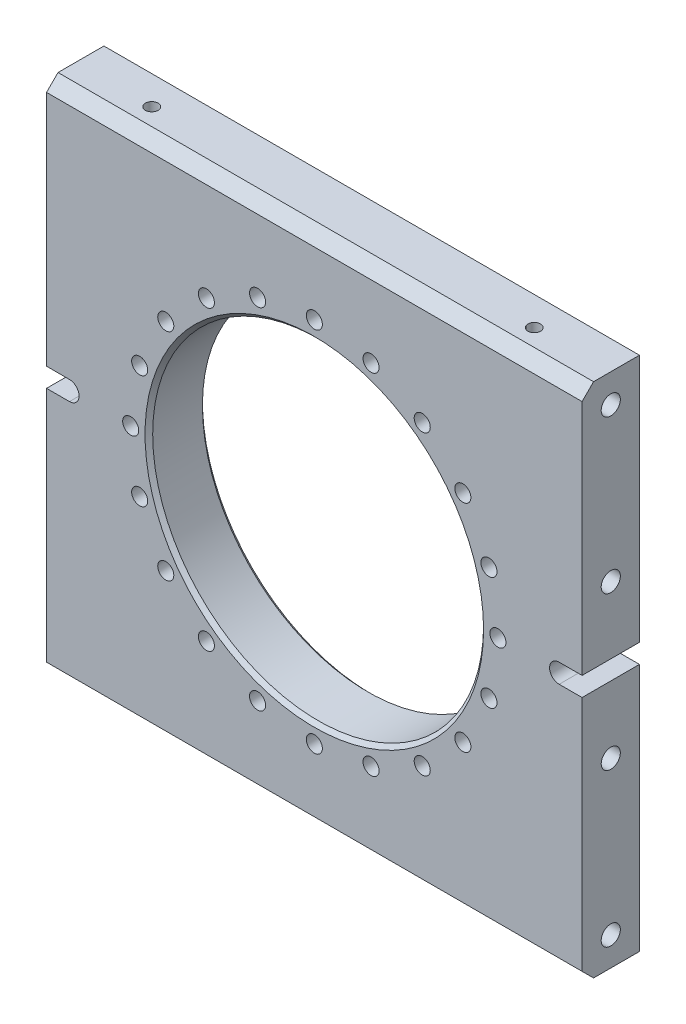
SolidWorks part; units mm, degrees
material "AL6061"
ref_plane "前视基准面" through (0, 0, 0) normal (0, 0, 1) x (1, 0, 0)
ref_plane "上视基准面" through (0, 0, 0) normal (0, 1, 0) x (1, 0, 0)
ref_plane "右视基准面" through (0, 0, 0) normal (1, 0, 0) x (0, 0, -1)
sketch "草图1" plane through (0, 0, 0) normal (0, 0, 1) x (1, 0, 0)
  line L0 (-78.7943, 0) -> (83.5001, 0) construction
  line L1 (0, 54.9642) -> (0, -73.3522) construction
  line L3 (-70, 67.5) -> (70, 67.5)
  line L4 (-70, 67.5) -> (-70, -67.5)
  line L5 (-70, -67.5) -> (70, -67.5)
  line L6 (70, 67.5) -> (70, -67.5)
  circle A0 centre (0, 0) radius 43.25
  dimension "D3" = 86.5
  dimension "D1" = 140
  dimension "D2" = 135
extrude "凸台-拉伸1" add sketch "草图1" along normal mid plane 15
hole_wizard "M6 螺纹孔1" positions "草图2" profile "草图3" tap size "M6" standard "GB"
sketch "草图2" plane through (70, 0, 0) normal (1, 0, 0) x (0, 0, -1)
  line L0 (-10.7947, 0) -> (15.8636, 0) construction
  line L1 (0, 71.0576) -> (0, -73.4981) construction
  point P0 (0, -20)
  point P2 (0, -60)
  point P11 (0, 60)
  point P12 (0, 20)
  dimension "D1" = 40
  dimension "D2" = 120
sketch "草图3" plane through (70, -20, 0) normal (0, 1, 0) x (0, 0, -1)
  line L0 (0, 0) -> (0, 19.5022)
  line L1 (0, 19.5022) -> (2.5, 18)
  line L2 (2.5, 18) -> (2.5, 0)
  line L5 (2.5, 0) -> (0, 0)
  line L10 (0, 19.5022) -> (-2.5, 18) construction
  line L11 (0, -6.35) -> (0, 107.95) construction
  dimension "螺纹孔钻头直径" = 5
  dimension "螺纹孔钻头深度" = 18
  dimension "导头角度" = 118
cosmetic thread "孔螺蚊线1" parameters "D1"=15, "D2"=6
cosmetic thread "孔螺蚊线2" parameters "D1"=15, "D2"=6
cosmetic thread "孔螺蚊线3" parameters "D1"=15, "D2"=6
cosmetic thread "孔螺蚊线4" parameters "D1"=15, "D2"=6
mirror "镜向2" about plane through (0, 0, 0) normal (1, 0, 0) of "M6 螺纹孔1"
hole_wizard "M5 螺纹孔1" positions "草图4" profile "草图5" tap size "M5" standard "GB" end condition through all
sketch "草图4" plane through (0, 0, 7.5) normal (0, 0, 1) x (1, 0, 0)
  line L0 (0, -4.0363) -> (0, 72.7472) construction
  line L1 (0, 0) -> (-73.1227, 0) construction
  circle A0 centre (0, 0) radius 48 construction
  point P0 (0, 48)
  dimension "D1" = 96
sketch "草图5" plane through (0, 48, 7.5) normal (1, 0, 0) x (0, -1, 0)
  line L0 (0, 0) -> (0, 15)
  line L1 (0, 15) -> (2.1, 15)
  line L2 (2.1, 15) -> (2.1, 0)
  line L5 (2.1, 0) -> (0, 0)
  line L11 (0, -6.35) -> (0, 107.95) construction
  dimension "通孔螺纹孔钻头直径" = 4.2
  dimension "通孔螺纹孔钻头深度" = 15
cosmetic thread "孔螺蚊线5" parameters "D2"=5
chamfer "倒角1" distance 1 angle 45 2 edges at (43.25, 0, -7.5) (43.25, 0, 7.5)
pattern_circular "阵列(圆周)1" count 20 over 360 about axis through (0, 0, 0) along (0, 0, 1) of "M5 螺纹孔1"
sketch "草图6" plane through (0, 0, 7.5) normal (0, 0, 1) x (1, 0, 0)
  line L0 (-71.7661, 0) -> (73.0925, 0) construction
  line L1 (0, 70.2589) -> (0, -69.4339) construction
  line L2 (70, -67.5) -> (70, 67.5) construction
  line L3 (70, 2.5) -> (64, 2.5)
  line L4 (70, 2.5) -> (70, -2.5)
  line L5 (70, -2.5) -> (64, -2.5)
  line L7 (-70, -2.5) -> (-64, -2.5)
  line L8 (-70, 2.5) -> (-70, -2.5)
  line L9 (-70, 2.5) -> (-64, 2.5)
  arc A0 (64, 2.5) -> (64, -2.5) centre (64, 0) ccw
  arc A1 (-64, 2.5) -> (-64, -2.5) centre (-64, 0) cw
  dimension "D2" = 6
  dimension "D1" = 5
extrude "切除-拉伸1" cut sketch "草图6" against normal through all
hole_wizard "M4 螺纹孔1" positions "草图7" profile "草图8" tap size "M4" standard "GB"
sketch "草图7" plane through (0, -67.5, 0) normal (0, -1, 0) x (-1, 0, 0)
  line L0 (0, 8.8808) -> (0, -13.9156) construction
  line L1 (-74.1931, 0) -> (74.4728, 0) construction
  point P0 (50, 0)
  point P9 (-50, 0)
  dimension "D1" = 100
sketch "草图8" plane through (-50, -67.5, 0) normal (1, 0, 0) x (0, 0, -1)
  line L0 (0, 0) -> (0, 18.0914)
  line L1 (0, 18.0914) -> (1.65, 17.1)
  line L2 (1.65, 17.1) -> (1.65, 0)
  line L5 (1.65, 0) -> (0, 0)
  line L10 (0, 18.0914) -> (-1.65, 17.1) construction
  line L11 (0, -6.35) -> (0, 107.95) construction
  dimension "螺纹孔钻头直径" = 3.3
  dimension "螺纹孔钻头深度" = 17.1
  dimension "导头角度" = 118
cosmetic thread "孔螺蚊线6" parameters "D1"=15, "D2"=4
cosmetic thread "孔螺蚊线7" parameters "D1"=15, "D2"=4
mirror "镜向3" about plane through (0, 0, 0) normal (0, 1, 0) of "M4 螺纹孔1"
chamfer "倒角2" distance 3 angle 45 2 edges at (0, 67.5, 7.5) (0, -67.5, 7.5)
